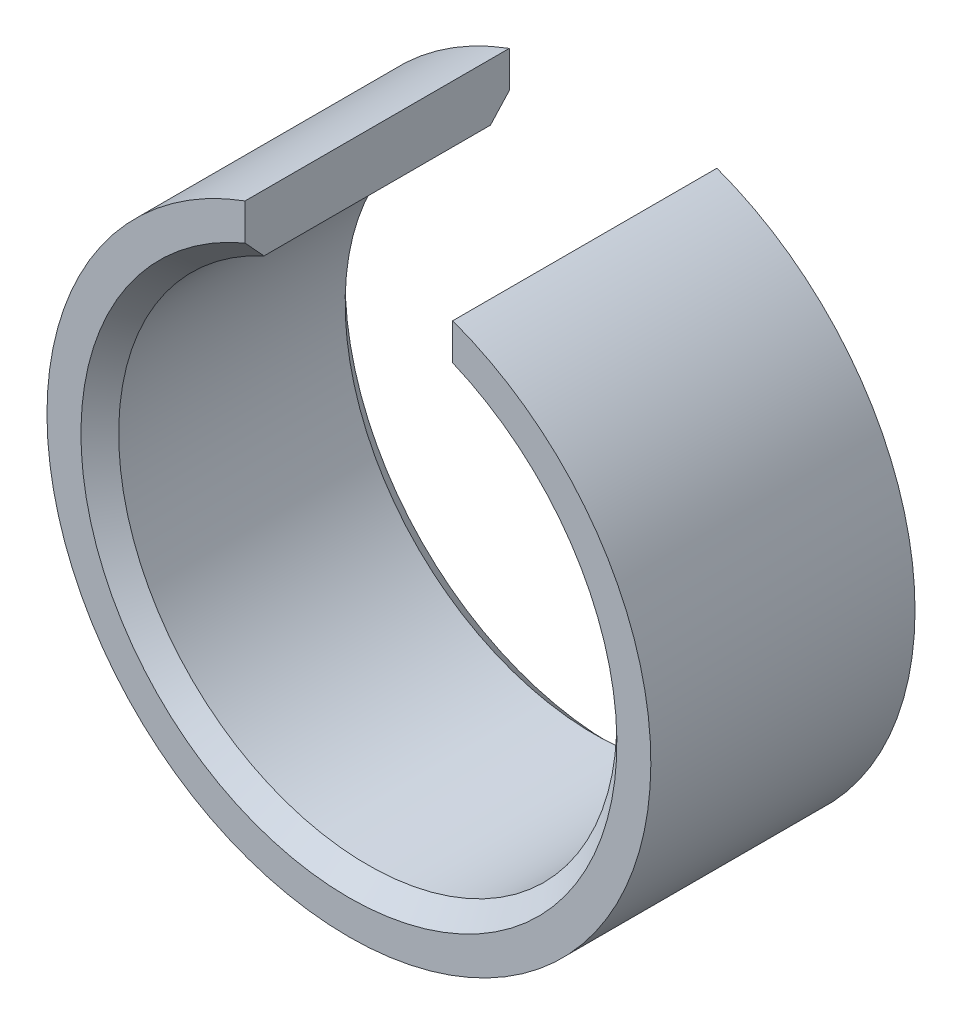
from build123d import *

# Parameters (mm, degrees)
SKETCH1_R           = 8
SKETCH1_R_2         = 6.6
BOSS_EXTRUDE1_DEPTH = 7
SKETCH2_W           = 5.5
SKETCH2_H           = 7.166353003
CUT_EXTRUDE1_DEPTH  = 14.304134696
CHAMFER1_SIZE       = 0.5


with BuildPart() as part:
    # Sketch1 → Boss-Extrude1 (new body)
    with BuildSketch(Plane.XY):
        Circle(SKETCH1_R)
        Circle(SKETCH1_R_2, mode=Mode.SUBTRACT)
    extrude(amount=BOSS_EXTRUDE1_DEPTH)

    # Sketch2 → Cut-Extrude1 (cut, through all)
    with BuildSketch(Plane.XY.offset(7)):
        with Locations((0, 7.454286829)):
            Rectangle(SKETCH2_W, SKETCH2_H)
    extrude(amount=-CUT_EXTRUDE1_DEPTH, mode=Mode.SUBTRACT)

    # Chamfer1
    chamfer1_edges = [part.edges().sort_by_distance(p)[0] for p in [
        (0, -6.6, 0),
        (0, -6.6, 7),
    ]]
    chamfer(chamfer1_edges, length=CHAMFER1_SIZE)


solid = part.part
